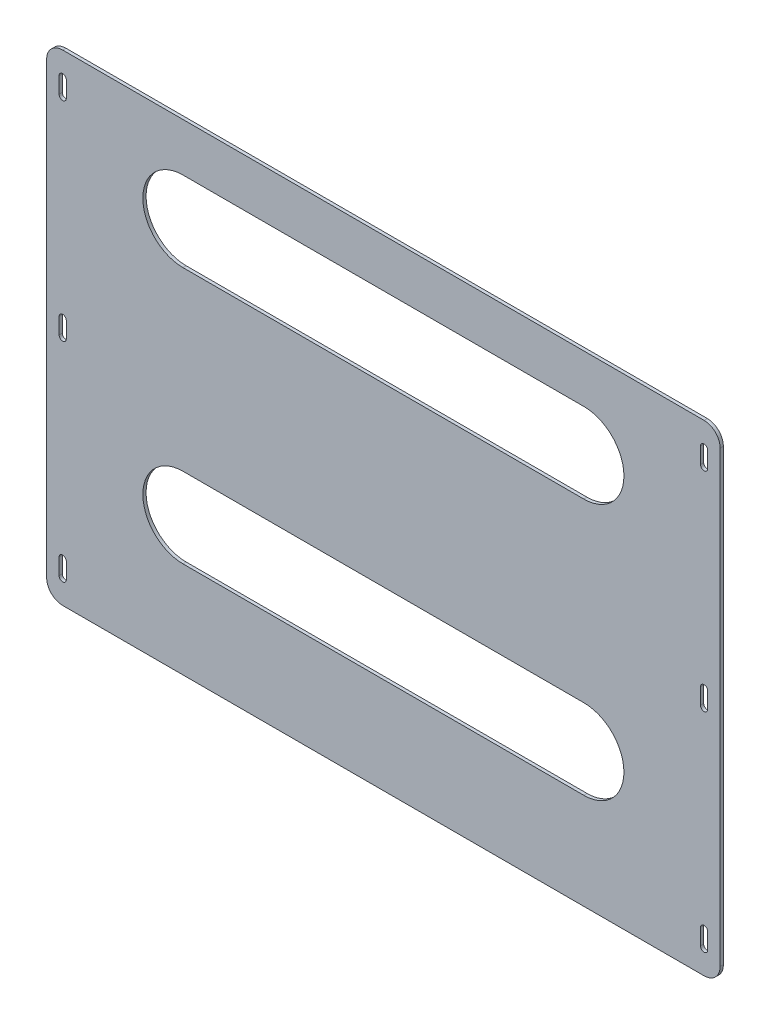
from build123d import *

# Parameters (mm, degrees)
SKETCH_1_W          = 420
SKETCH_1_H          = 300
EXTRUDE_1_DEPTH     = 2
HOLE_WIZARD_M4_2_D  = 3.3
CUT_EXTRUDE_1_DEPTH = 10
FILLET_1_R          = 10
CUT_EXTRUDE_2_DEPTH = 10


with BuildPart() as part:
    # 草图1 → 凸台-拉伸1 (new body)
    with BuildSketch(Plane.XY):
        Rectangle(SKETCH_1_W, SKETCH_1_H)
    extrude(amount=EXTRUDE_1_DEPTH)

    # M4 螺纹孔的螺纹孔钻头2 (through all)
    with Locations(Plane.XY.offset(2)):
        with Locations((200, 0), (-200, -130), (-200, 0), (200, -130)):
            Hole(HOLE_WIZARD_M4_2_D / 2)

    # 草图4 → 切除-拉伸1 (cut)
    with BuildSketch(Plane.XY.offset(2)):
        with BuildLine():
            Line((197.75, -135), (197.75, -125))
            ThreePointArc((197.75, -125), (200, -122.75), (202.25, -125))
            Line((202.25, -125), (202.25, -135))
            ThreePointArc((202.25, -135), (200, -137.25), (197.75, -135))
        make_face()
        with BuildLine():
            Line((-197.75, -135), (-197.75, -125))
            ThreePointArc((-197.75, -125), (-200, -122.75), (-202.25, -125))
            Line((-202.25, -125), (-202.25, -135))
            ThreePointArc((-202.25, -135), (-200, -137.25), (-197.75, -135))
        make_face()
        with BuildLine():
            Line((202.25, -5), (202.25, 5))
            ThreePointArc((202.25, 5), (200, 7.25), (197.75, 5))
            Line((197.75, 5), (197.75, -5))
            ThreePointArc((197.75, -5), (200, -7.25), (202.25, -5))
        make_face()
        with BuildLine():
            Line((197.75, 135), (197.75, 125))
            ThreePointArc((197.75, 125), (200, 122.75), (202.25, 125))
            Line((202.25, 125), (202.25, 135))
            ThreePointArc((202.25, 135), (200, 137.25), (197.75, 135))
        make_face()
        with BuildLine():
            Line((-197.75, 135), (-197.75, 125))
            ThreePointArc((-197.75, 125), (-200, 122.75), (-202.25, 125))
            Line((-202.25, 125), (-202.25, 135))
            ThreePointArc((-202.25, 135), (-200, 137.25), (-197.75, 135))
        make_face()
        with BuildLine():
            Line((-202.25, -5), (-202.25, 5))
            ThreePointArc((-202.25, 5), (-200, 7.25), (-197.75, 5))
            Line((-197.75, 5), (-197.75, -5))
            ThreePointArc((-197.75, -5), (-200, -7.25), (-202.25, -5))
        make_face()
    extrude(amount=-CUT_EXTRUDE_1_DEPTH, mode=Mode.SUBTRACT)

    # 圆角1
    fillet_1_edges = [part.edges().sort_by_distance(p)[0] for p in [
        (210, -150, 1),
        (-210, -150, 1),
        (-210, 150, 1),
        (210, 150, 1),
    ]]
    fillet(fillet_1_edges, radius=FILLET_1_R)

    # 草图5 → 切除-拉伸2 (cut)
    with BuildSketch(Plane.XY.offset(2)):
        with BuildLine():
            Line((-125, -40), (125, -40))
            ThreePointArc((125, -40), (150, -65), (125, -90))
            Line((125, -90), (-125, -90))
            ThreePointArc((-125, -90), (-150, -65), (-125, -40))
        make_face()
        with BuildLine():
            Line((125, 70), (-125, 70))
            ThreePointArc((-125, 70), (-150, 95), (-125, 120))
            Line((-125, 120), (125, 120))
            ThreePointArc((125, 120), (150, 95), (125, 70))
        make_face()
    extrude(amount=-CUT_EXTRUDE_2_DEPTH, mode=Mode.SUBTRACT)


solid = part.part
